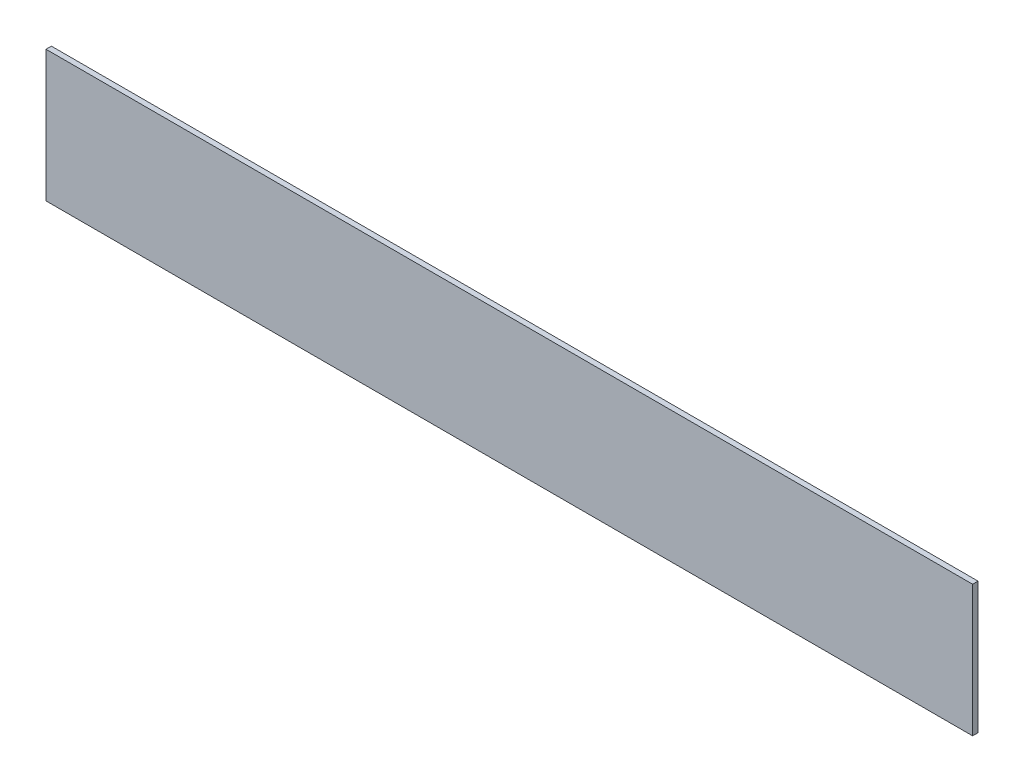
SolidWorks part; units mm, degrees
ref_plane "Frontal" through (0, 0, 0) normal (0, 0, 1) x (1, 0, 0)
ref_plane "Superior" through (0, 0, 0) normal (0, 1, 0) x (1, 0, 0)
ref_plane "Direito" through (0, 0, 0) normal (1, 0, 0) x (0, 0, -1)
sketch "Sketch1" plane through (0, 0, 0) normal (0, 0, 1) x (1, 0, 0)
  line L1 (-257.5, 36.5) -> (257.5, 36.5)
  line L2 (-257.5, 36.5) -> (-257.5, -36.5)
  line L3 (-257.5, -36.5) -> (257.5, -36.5)
  line L4 (257.5, 36.5) -> (257.5, -36.5)
  line L5 (-257.5, 36.5) -> (257.5, -36.5) construction
  line L6 (-257.5, -36.5) -> (257.5, 36.5) construction
  point P0 (0, 0)
  dimension "D1" = 73
  dimension "D2" = 515
extrude "Boss-Extrude1" add sketch "Sketch1" along normal blind 3
